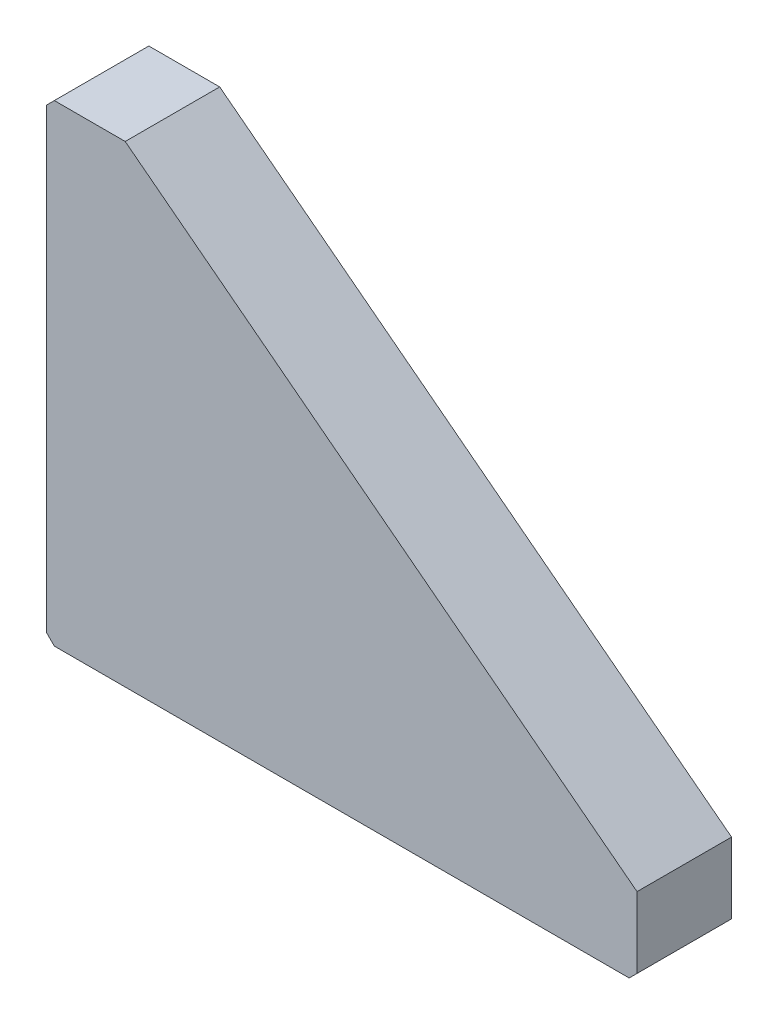
SolidWorks part; units mm, degrees
material "AL6061"
ref_plane "Front" through (0, 0, 0) normal (0, 0, 1) x (1, 0, 0)
ref_plane "Top" through (0, 0, 0) normal (0, 1, 0) x (1, 0, 0)
ref_plane "Right" through (0, 0, 0) normal (1, 0, 0) x (0, 0, -1)
sketch "Sketch1" plane through (0, 0, 0) normal (0, 0, 1) x (1, 0, 0)
  line L1 (-37.5, 30) -> (37.5, 30)
  line L2 (-37.5, 30) -> (-37.5, -30)
  line L3 (-37.5, -30) -> (37.5, -30)
  line L4 (37.5, 30) -> (37.5, -30)
  line L5 (-37.5, 30) -> (37.5, -30) construction
  line L6 (-37.5, -30) -> (37.5, 30) construction
  point P0 (0, 0)
  dimension "D1" = 60
  dimension "D2" = 75
extrude "Boss-Extrude1" add sketch "Sketch1" along normal mid plane 12
sketch "Sketch2" plane through (0, 0, 6) normal (0, 0, 1) x (1, 0, 0)
  line L0 (-27.5, 30) -> (37.5, -20)
  line L1 (37.5, -30) -> (37.5, 30) construction
  line L2 (37.5, -20) -> (37.5, 30)
  line L3 (37.5, 30) -> (-37.5, 30) construction
  line L4 (37.5, 30) -> (-27.5, 30)
  line L5 (-37.5, 30) -> (-37.5, -30) construction
  line L6 (-37.5, -30) -> (37.5, -30) construction
  dimension "D1" = 10
  dimension "D2" = 10
extrude "Cut-Extrude1" cut sketch "Sketch2" against normal through all
hole_wizard "M6 Tapped Hole1" positions "Sketch5" profile "Sketch7" tap size "M6" standard "ISO"
sketch "Sketch5" plane through (-37.5, 0, 0) normal (-1, 0, 0) x (0, 0, 1)
  line L0 (6, -30) -> (-6, -30) construction
  line L1 (6, 30) -> (-6, 30) construction
  point P0 (0, 20)
  point P2 (0, -15)
  dimension "D1" = 15
  dimension "D2" = 10
sketch "Sketch7" plane through (-37.5, 20, 0) normal (0, 1, 0) x (0, 0, 1)
  line L0 (0, 0) -> (0, 13.5022)
  line L1 (0, 13.5022) -> (2.5, 12)
  line L2 (2.5, 12) -> (2.5, 0)
  line L5 (2.5, 0) -> (0, 0)
  line L10 (0, 13.5022) -> (-2.5, 12) construction
  line L11 (0, -6.35) -> (0, 107.95) construction
  dimension "螺纹孔钻头直径" = 5
  dimension "螺纹孔钻头深度" = 12
  dimension "导头角度" = 118
cosmetic thread "Cosmetic Thread1" parameters "D1"=12, "D2"=6
cosmetic thread "Cosmetic Thread2" parameters "D1"=12, "D2"=6
hole_wizard "M6 Tapped Hole2" positions "Sketch8" profile "Sketch9" tap size "M6" standard "ISO"
sketch "Sketch8" plane through (0, -30, 0) normal (0, -1, 0) x (-1, 0, 0)
  line L0 (37.5, -6) -> (37.5, 6) construction
  line L1 (-37.5, -6) -> (-37.5, 6) construction
  point P0 (22.5, 0)
  point P2 (-27.5, 0)
  dimension "D1" = 15
  dimension "D2" = 10
sketch "Sketch9" plane through (-22.5, -30, 0) normal (1, 0, 0) x (0, 0, -1)
  line L0 (0, 0) -> (0, 16.5022)
  line L1 (0, 16.5022) -> (2.5, 15)
  line L2 (2.5, 15) -> (2.5, 0)
  line L5 (2.5, 0) -> (0, 0)
  line L10 (0, 16.5022) -> (-2.5, 15) construction
  line L11 (0, -6.35) -> (0, 107.95) construction
  dimension "螺纹孔钻头直径" = 5
  dimension "螺纹孔钻头深度" = 15
  dimension "导头角度" = 118
cosmetic thread "Cosmetic Thread3" parameters "D1"=12, "D2"=6
cosmetic thread "Cosmetic Thread4" parameters "D1"=12, "D2"=6
chamfer "Chamfer1" distance 1 angle 45 3 edges at (-37.5, 30, 0) (37.5, -30, 0) (-37.5, -30, 0)
